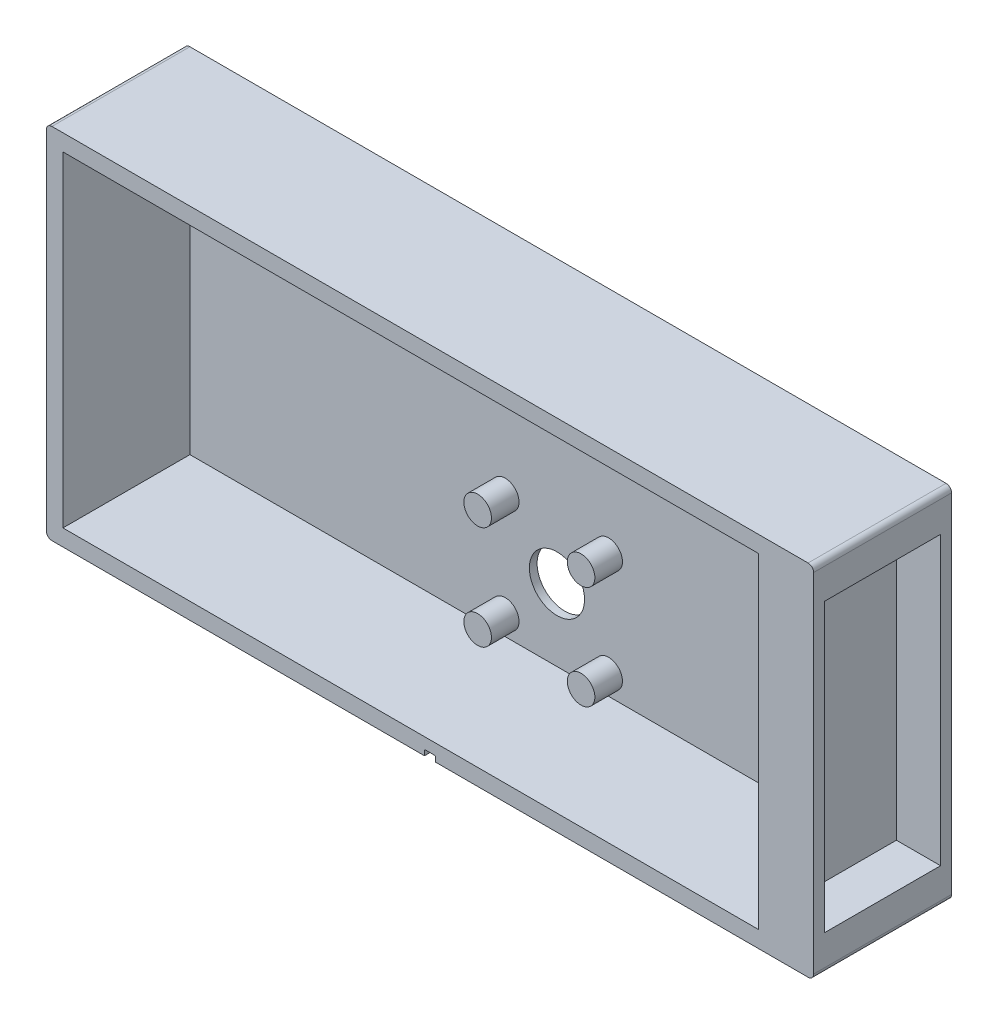
SolidWorks part; units mm, degrees
ref_plane "Front Plane" through (0, 0, 0) normal (0, 0, 1) x (1, 0, 0)
ref_plane "Top Plane" through (0, 0, 0) normal (0, 1, 0) x (1, 0, 0)
ref_plane "Right Plane" through (0, 0, 0) normal (1, 0, 0) x (0, 0, -1)
other "Configuration Table"
sketch "Sketch1" plane through (0, 0, 0) normal (0, 0, 1) x (1, 0, 0)
  line L1 (-68.5, 32.5) -> (68.5, 32.5)
  line L2 (-69.5, 31.5) -> (-69.5, -31.5)
  line L3 (-68.5, -32.5) -> (68.5, -32.5)
  line L4 (69.5, 31.5) -> (69.5, -31.5)
  line L5 (-69.5, 32.5) -> (69.5, -32.5) construction
  line L6 (-69.5, -32.5) -> (69.5, 32.5) construction
  arc A0 (-69.5, -31.5) -> (-68.5, -32.5) centre (-68.5, -31.5) ccw
  arc A1 (68.5, -32.5) -> (69.5, -31.5) centre (68.5, -31.5) ccw
  arc A2 (68.5, 32.5) -> (69.5, 31.5) centre (68.5, 31.5) cw
  arc A3 (-68.5, 32.5) -> (-69.5, 31.5) centre (-68.5, 31.5) ccw
  point P0 (0, 0)
  dimension "D3" = 1
  dimension "D1" = 139
  dimension "D2" = 65
extrude "Boss-Extrude1" add sketch "Sketch1" along normal blind 25
shell "Shell1" thickness 2
sketch "Sketch6" plane through (0, 0, 0) normal (0, 0, -1) x (-1, 0, 0)
  line L0 (68.5, -32.5) -> (-68.5, -32.5) construction
  circle A0 centre (0, -16.5) radius 10.15
  dimension "D1" = 20.3
  dimension "D2" = 16
extrude "Cut-Extrude3" cut sketch "Sketch6" against normal blind 0.6
sketch "Sketch10" plane through (0, 0, 0.6) normal (0, 0, -1) x (-1, 0, 0)
  circle A0 centre (0, -16.5) radius 5
  dimension "D1" = 10
extrude "Cut-Extrude4" cut sketch "Sketch10" against normal through all
sketch "Sketch11" plane through (0, 0, 0.6) normal (0, 0, -1) x (-1, 0, 0)
  circle A0 centre (0, -16.5) radius 7
  circle A2 centre (0, -16.5) radius 8
  dimension "D1" = 16
  dimension "D2" = 14
extrude "Boss-Extrude5" add sketch "Sketch11" along normal blind 0.6
sketch "Sketch13" plane through (0, 0, 2) normal (0, 0, 1) x (1, 0, 0)
  line L0 (0, -16.5) -> (0, 0) construction
  line L1 (0, -16.5) -> (-9.3692, -7.1308) construction
  circle A0 centre (0, -16.5) radius 13.25 construction
  circle A1 centre (-9.3692, -7.1308) radius 2.5
  circle A2 centre (9.3692, -7.1308) radius 2.5
  circle A3 centre (9.3692, -25.8692) radius 2.5
  circle A4 centre (-9.3692, -25.8692) radius 2.5
  circle A5 centre (0, -16.5) radius 5 construction
  point P16 (0, -16.5)
  dimension "D1" = 26.5
  dimension "D3" = 5
  dimension "D2" = 45
  dimension "D4" = 4
extrude "Boss-Extrude6" add sketch "Sketch13" along normal blind 5
sketch "Sketch15" plane through (0, 0, 7) normal (0, 0, 1) x (1, 0, 0)
  circle A0 centre (9.3692, -7.1308) radius 0.5
  circle A1 centre (-9.3692, -7.1308) radius 0.5
  circle A2 centre (-9.3692, -25.8692) radius 0.5
  circle A3 centre (9.3692, -25.8692) radius 0.5
  dimension "D1" = 1
extrude "Cut-Extrude5" cut sketch "Sketch15" against normal through all from offset 2 offset against normal yes
sketch "Sketch16" plane through (0, -32.5, 0) normal (0, -1, 0) x (-1, 0, 0)
  line L1 (1, 29.0822) -> (-1, 29.0822)
  line L2 (1, 29.0822) -> (1, -29.0822)
  line L3 (1, -29.0822) -> (-1, -29.0822)
  line L4 (-1, 29.0822) -> (-1, -29.0822)
  line L5 (1, 29.0822) -> (-1, -29.0822) construction
  line L6 (1, -29.0822) -> (-1, 29.0822) construction
  point P0 (0, 0)
  dimension "D1" = 2
extrude "Cut-Extrude6" cut sketch "Sketch16" against normal blind 1
fillet "Fillet2" radius 0.1 4 edges at (-7, -16.5, 0) (-8, -16.5, 0) (-7, -16.5, 0.6) (-8, -16.5, 0.6)
sketch "Sketch17" plane through (0, 0, 0) normal (0, 0, -1) x (-1, 0, 0)
  circle A0 centre (0, -16.5) radius 15.5
  circle A1 centre (0, -16.5) radius 10.15
  circle A2 centre (-9.3692, -7.1308) radius 0.5
  circle A3 centre (9.3692, -7.1308) radius 0.5
  circle A4 centre (9.3692, -25.8692) radius 0.5
  circle A5 centre (-9.3692, -25.8692) radius 0.5
  dimension "D1" = 31
  dimension "D2" = 1
  dimension "D3" = 20.3
extrude "Boss-Extrude7" add sketch "Sketch17" along normal blind 1.2
sketch "Sketch18" plane through (0, -32.5, 0) normal (0, -1, 0) x (-1, 0, 0)
  line L1 (1, 0) -> (-1, 0)
  line L2 (1, 0) -> (1, 1.6262)
  line L3 (1, 1.6262) -> (-1, 1.6262)
  line L4 (-1, 0) -> (-1, 1.6262)
  dimension "D1" = 2
extrude "Cut-Extrude7" cut sketch "Sketch18" against normal blind 1
fillet "Fillet3" radius 0.5 1 edges at (0, -1, 0)
fillet "Fillet5" radius 0.2 2 edges at (1, -31.5, 11.9) (-1, -31.5, 11.9)
sketch "Sketch21" plane through (0, 0, 2) normal (0, 0, 1) x (1, 0, 0)
  line L0 (-66.5, 29.5) -> (-66.5, -29.5)
  line L1 (-67.5, 30.5) -> (67.5, 30.5)
  line L2 (-67.5, 30.5) -> (-67.5, -30.5)
  line L3 (-67.5, -30.5) -> (67.5, -30.5)
  line L4 (67.5, 30.5) -> (67.5, -30.5)
  line L5 (-66.5, -29.5) -> (66.5, -29.5)
  line L6 (66.5, 29.5) -> (66.5, -29.5)
  line L7 (-66.5, 29.5) -> (66.5, 29.5)
  dimension "D1" = 1
extrude "Boss-Extrude8" add sketch "Sketch21" along normal blind 23
sketch "Sketch20" plane through (69.5, 0, 0) normal (1, 0, 0) x (0, 0, -1)
  line L0 (0, 0) -> (-25, 0) construction
  line L1 (-25, -31.5) -> (-25, 31.5) construction
  line L2 (0, -31.5) -> (0, 31.5) construction
  line L3 (-23, 26) -> (-2, 26)
  line L4 (-23, 26) -> (-23, -26)
  line L5 (-23, -26) -> (-2, -26)
  line L6 (-2, 26) -> (-2, -26)
  line L7 (-23, 26) -> (-2, -26) construction
  line L8 (-23, -26) -> (-2, 26) construction
  point P5 (-12.5, 0)
  dimension "D1" = 21
  dimension "D2" = 52
  dimension "D3" = 2
extrude "Cut-Extrude8" cut sketch "Sketch20" against normal up to next
sketch "Sketch22" plane through (66.5, 0, 0) normal (-1, 0, 0) x (0, 0, 1)
  line L0 (25, -29.5) -> (25, 29.5) construction
  line L1 (2, 26) -> (23, 26)
  line L2 (2, 26) -> (2, -26)
  line L3 (2, -26) -> (23, -26)
  line L4 (23, 26) -> (23, -26)
  line L5 (25, 30.0757) -> (0.3876, 30.0757)
  line L6 (25, 30.0757) -> (25, -30.4661)
  line L7 (25, -30.4661) -> (0.3876, -30.4661)
  line L8 (0.3876, 30.0757) -> (0.3876, -30.4661)
extrude "Boss-Extrude9" add sketch "Sketch22" along normal blind 7
sketch "Sketch23" plane through (59.5, 0, 0) normal (-1, 0, 0) x (0, 0, 1)
  line L1 (23.7407, 26.9818) -> (0.9725, 26.9818)
  line L2 (23.7407, 26.9818) -> (23.7407, -27.3611)
  line L3 (23.7407, -27.3611) -> (0.9725, -27.3611)
  line L4 (0.9725, 26.9818) -> (0.9725, -27.3611)
extrude "Boss-Extrude12" add sketch "Sketch23" against normal blind 2
